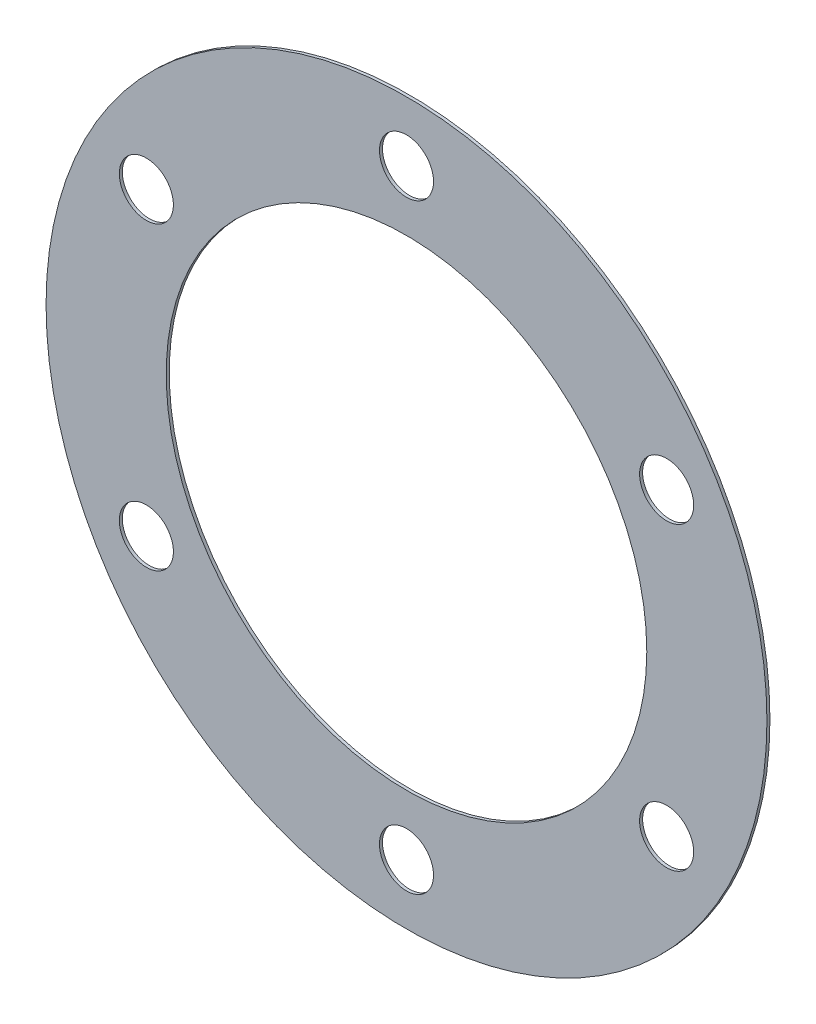
SolidWorks part; units mm, degrees
ref_plane "Front Plane" through (0, 0, 0) normal (0, 0, 1) x (1, 0, 0)
ref_plane "Top Plane" through (0, 0, 0) normal (0, 1, 0) x (1, 0, 0)
ref_plane "Right Plane" through (0, 0, 0) normal (1, 0, 0) x (0, 0, -1)
sketch "Sketch1" plane through (0, 0, 0) normal (0, 0, 1) x (1, 0, 0)
  circle A0 centre (0, 0) radius 40
  circle A1 centre (0, 0) radius 60
  dimension "D1" = 80
  dimension "D2" = 120
extrude "Boss-Extrude1" add sketch "Sketch1" along normal blind 0.5
sketch "Sketch2" plane through (0, 0, 0.5) normal (0, 0, 1) x (1, 0, 0)
  circle A0 centre (0, 50) radius 4.5
  dimension "D2" = 9
  dimension "D1" = 50
extrude "Cut-Extrude1" cut sketch "Sketch2" against normal through all
pattern_circular "CirPattern1" count 6 over 360 about axis through (0, 0, 0) along (0, 0, 1) of "Cut-Extrude1"
